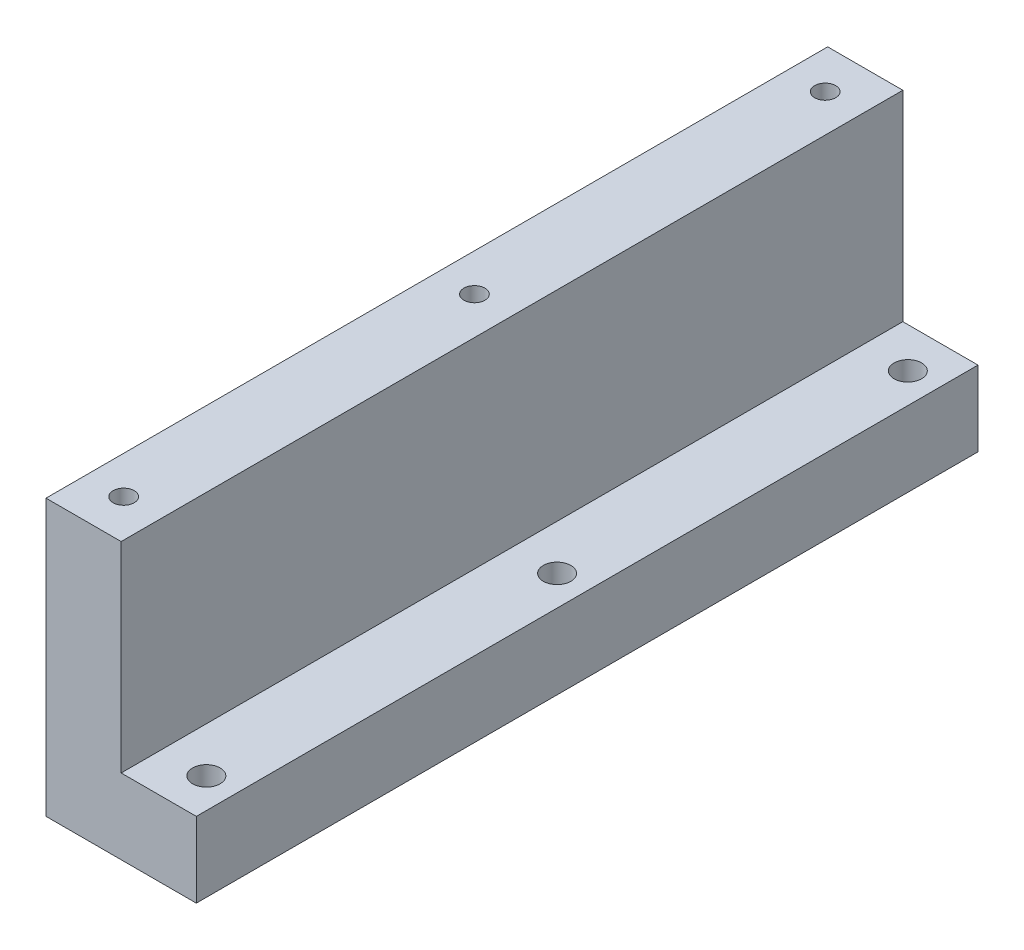
from build123d import *

# Parameters (mm, degrees)
EXTRUDE1_DEPTH        = 78
M5_TAPPED_HOLE1_D     = 4.2
M5_TAPPED_HOLE1_DEPTH = 14.4
M5_TAPPED_HOLE1_TIP   = 1.2618073
SKETCH3_R             = 2.75
CUT_EXTRUDE1_DEPTH    = 93.649878575


with BuildPart() as part:
    # Sketch1 → Extrude1 (new, symmetric)
    with BuildSketch(Plane.XY):
        Polygon((0, 55), (0, 0), (30, 0), (30, 15), (15, 15), (15, 55), align=None)
    extrude(amount=EXTRUDE1_DEPTH, both=True)

    # M5 Tapped Hole1
    with Locations(Plane(origin=(7.5, 55, 0), x_dir=(0, 0, 1), z_dir=(0, 1, 0))):
        with Locations((0, 0), (-70, 0), (70, 0)):
            Hole(M5_TAPPED_HOLE1_D / 2, depth=M5_TAPPED_HOLE1_DEPTH)
            with Locations((0, 0, -(M5_TAPPED_HOLE1_DEPTH + M5_TAPPED_HOLE1_TIP / 2))):  # 118° drill point
                Cone(0, M5_TAPPED_HOLE1_D / 2, M5_TAPPED_HOLE1_TIP, mode=Mode.SUBTRACT)

    # Sketch3 → Cut-Extrude1 (cut, through all)
    with BuildSketch(Plane(origin=(0, 15, 0), x_dir=(1, 0, 0), z_dir=(0, 1, 0))):
        with Locations(Location((24, 0, 0), (0, 0, 270))):
            Circle(SKETCH3_R)
        with Locations(Location((24, 70, 0), (0, 0, 270))):
            Circle(SKETCH3_R)
        with Locations(Location((24, -70, 0), (0, 0, 90))):
            Circle(SKETCH3_R)
    extrude(amount=-CUT_EXTRUDE1_DEPTH, mode=Mode.SUBTRACT)


solid = part.part
